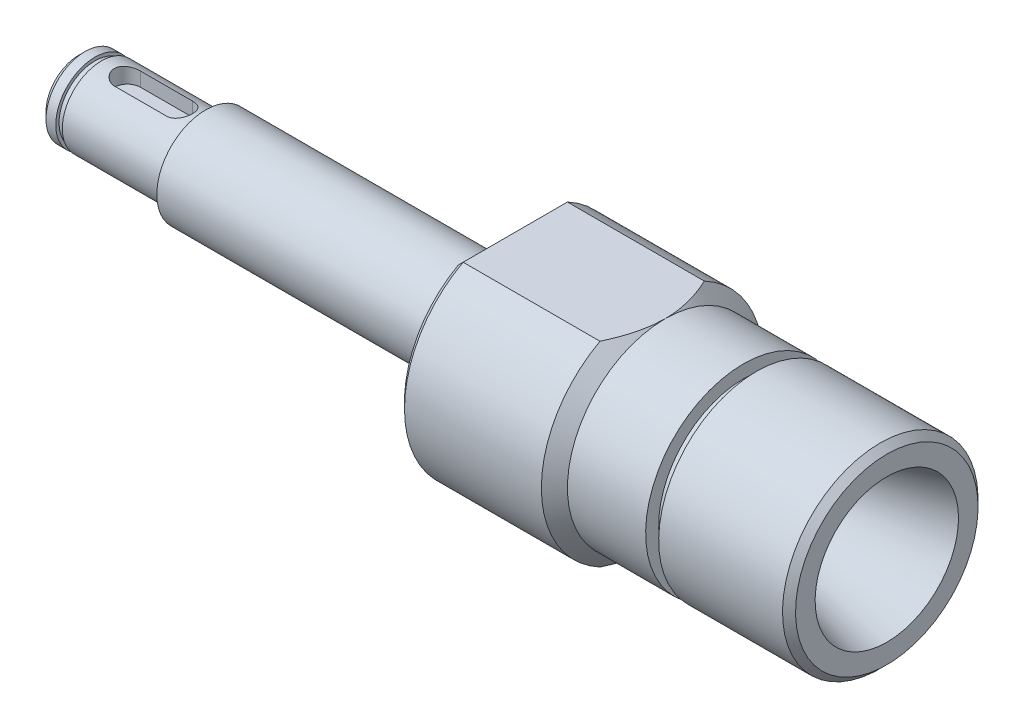
from build123d import *

# Parameters (mm, degrees)
CUT_EXTRUDE1_START = 3.5
CUT_EXTRUDE1_DEPTH = 10
CUT_EXTRUDE2_REACH = 72.242
CHAMFER1_SIZE      = 1
CHAMFER2_SIZE      = 1


with BuildPart() as part:
    # Sketch1 → Revolve1 (revolve)
    with BuildSketch(Plane.XY):
        Polygon((0, 0), (0, 6), (2.5, 6), (2.5, 5.5), (3.5, 5.5), (3.5, 6), (18.5, 6), (18.5, 5.5), (19.5, 5.5), (19.5, 7.5), (64, 7.5), (64, 6.5), (66, 6.5), (66, 17), (88, 17), (90, 15), (102, 15), (102, 13), (104, 13), (104, 15), (124, 15), (124, 0), align=None)
    revolve(axis=Axis((124, 0, 0), (-1, 0, 0)))

    # Sketch3 → Cut-Extrude1 (cut)
    with BuildSketch(Plane(origin=(0, 0, 0), x_dir=(1, 0, 0), z_dir=(0, 1, 0)).offset(CUT_EXTRUDE1_START)):
        with BuildLine():
            Line((15.5, -2), (7.5, -2))
            ThreePointArc((7.5, -2), (5.5, 0), (7.5, 2))
            Line((7.5, 2), (15.5, 2))
            ThreePointArc((15.5, 2), (17.5, 0), (15.5, -2))
        make_face()
    extrude(amount=CUT_EXTRUDE1_DEPTH, mode=Mode.SUBTRACT)

    # Cut-Extrude2: up to this cone (the profile starts inside it)
    cut_extrude2_end = Plane(origin=(66, 0, 0), z_dir=(-1, 0, 0)).offset(-38.999999) * Cone(1e-06, 150.742, 150.741999, align=(Align.CENTER, Align.CENTER, Align.MIN), mode=Mode.PRIVATE)
    # Sketch6 → Cut-Extrude2 (cut, up to the surface)
    with BuildSketch(Plane.ZY.offset(-66), mode=Mode.PRIVATE) as cut_extrude2_sk1:
        with BuildLine():
            Line((-8, 15), (8, 15))
            ThreePointArc((8, 15), (0, 17), (-8, 15))
        make_face()
    cut_extrude2_tool1 = extrude(cut_extrude2_sk1.sketch, amount=-CUT_EXTRUDE2_REACH, mode=Mode.PRIVATE) & cut_extrude2_end
    add(cut_extrude2_tool1.solids().sort_by_distance((66, 15.804176, 0))[0], mode=Mode.SUBTRACT)
    # Sketch6 → Cut-Extrude2 (cut, up to the surface)
    with BuildSketch(Plane.ZY.offset(-66), mode=Mode.PRIVATE) as cut_extrude2_sk2:
        with BuildLine():
            Line((-8, -15), (8, -15))
            ThreePointArc((8, -15), (0, -17), (-8, -15))
        make_face()
    cut_extrude2_tool2 = extrude(cut_extrude2_sk2.sketch, amount=-CUT_EXTRUDE2_REACH, mode=Mode.PRIVATE) & cut_extrude2_end
    add(cut_extrude2_tool2.solids().sort_by_distance((66, -15.804176, 0))[0], mode=Mode.SUBTRACT)

    # Chamfer1
    chamfer1_edges = [part.edges().sort_by_distance(p)[0] for p in [
        (124, -15, 0),
        (66, 0, 17),
        (0, -6, 0),
        (66, 0, -17),
        (66, 15, 0),
        (66, -15, 0),
    ]]
    chamfer(chamfer1_edges, length=CHAMFER1_SIZE)

    # Sketch7 → Cut-Revolve1 (revolve, cut)
    with BuildSketch(Plane.XY, mode=Mode.PRIVATE) as cut_revolve1_sk:
        Polygon((124, 11), (108, 6.712812921), (108, 9.5), (103, 9.5), (103, 9), (97, 9), (97, 9.5), (92, 9.5), (92, 7), (76, 7), (71.958548116, 0), (124, 0), align=None)
    revolve(cut_revolve1_sk.sketch.rotate(Axis((71.958548116, 0, 0), (1, 0, 0)), 180), axis=Axis((71.958548116, 0, 0), (1, 0, 0)), mode=Mode.SUBTRACT)

    # Chamfer2
    chamfer2_edges = [part.edges().sort_by_distance(p)[0] for p in [
        (92, 7, 0),
    ]]
    chamfer(chamfer2_edges, length=CHAMFER2_SIZE)


solid = part.part
